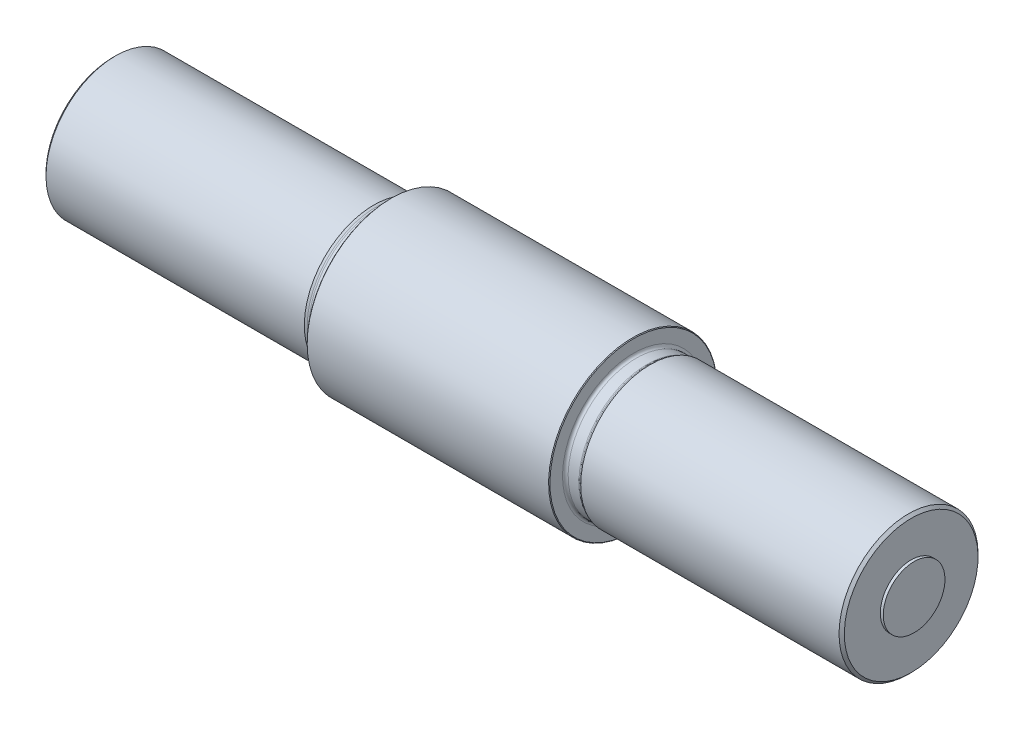
SolidWorks part; units mm, degrees
material "42CrMo"
ref_plane "Front plane" through (0, 0, 0) normal (0, 0, 1) x (1, 0, 0)
ref_plane "Top plane" through (0, 0, 0) normal (0, 1, 0) x (1, 0, 0)
ref_plane "Right plane" through (0, 0, 0) normal (1, 0, 0) x (0, 0, -1)
sketch "Sketch1" plane through (0, 0, 0) normal (0, 0, 1) x (1, 0, 0)
  line L0 (0, 45.5978) -> (0, -37.6046) construction
  line L1 (-580.619, 0) -> (79.7507, 0) construction
  line L2 (137.3251, 95.2119) -> (-137.3251, 95.2119)
  line L3 (-137.3251, 95.2119) -> (-137.3251, 77.0001)
  line L4 (-137.3251, 77.0001) -> (-153.5485, 77.0001)
  line L5 (-153.5485, 77.0001) -> (-156.3751, 78.632)
  line L6 (-156.3751, 78.632) -> (-451.6501, 78.632)
  line L7 (-451.6501, 78.632) -> (-451.6501, 34.925)
  line L8 (451.6501, 78.6321) -> (451.6501, 34.925)
  line L9 (156.3751, 78.6321) -> (451.6501, 78.6321)
  line L10 (153.5485, 77.0001) -> (156.3751, 78.6321)
  line L11 (137.3251, 77.0001) -> (153.5485, 77.0001)
  line L12 (137.3251, 95.2119) -> (137.3251, 77.0001)
  line L13 (-454.9521, 0) -> (454.9521, 0)
  line L14 (-451.6501, 34.925) -> (-454.9521, 34.925)
  line L15 (-454.9521, 34.925) -> (-454.9521, 0)
  line L16 (454.9521, 34.925) -> (454.9521, 0)
  line L17 (451.6501, 34.925) -> (454.9521, 34.925)
  point P13 (0, 95.2119)
  dimension "D1" = 190.4238
  dimension "D2" = 154.0002
  dimension "D3" = 157.2641
  dimension "D4" = 314.325
  dimension "D5" = 30
  dimension "D6" = 274.6502
  dimension "D7" = 19.05
  dimension "D8" = 903.3002
  dimension "D9" = 69.85
  dimension "D10" = 3.302
revolve "Revolve1" add sketch "Sketch1" angle 360 about L13
chamfer "Chamfer1" distance 3 angle 45 2 edges at (451.6501, -78.632, 0) (-451.6501, -78.632, 0)
chamfer "Chamfer2" distance 0.762 angle 45 2 edges at (137.3251, -95.2119, 0) (-137.3251, -95.2119, 0)
fillet "Fillet1" radius 3.175 4 edges at (153.5485, -77.0001, 0) (137.3251, -77.0001, 0) (-153.5485, -77.0001, 0) (-137.3251, -77.0001, 0)
ref_plane "Plane1" through (0, 0, -95.2119) normal (0, 0, -1) x (0, -1, 0)
sketch "Sketch2" plane through (0, 0, -95.2119) normal (0, 0, -1) x (0, -1, 0)
  circle A0 centre (0, 0) radius 11.3157
  dimension "D1" = 22.6314
extrude "Cut-Extrude1" cut sketch "Sketch2" against normal blind 28.702
